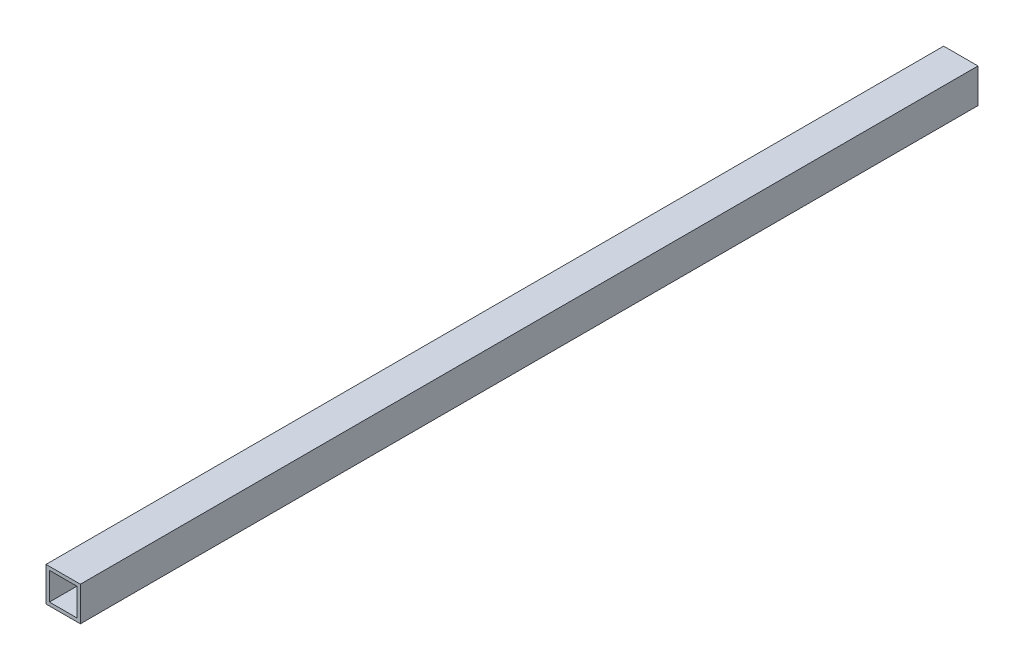
from build123d import *

# Parameters (mm, degrees)
SKETCH1_W           = 30
SKETCH1_H           = 30
SKETCH1_W_2         = 24
SKETCH1_H_2         = 24
BOSS_EXTRUDE2_DEPTH = 784


with BuildPart() as part:
    # Sketch1 → Boss-Extrude2 (new body)
    with BuildSketch(Plane.XY):
        with Locations((-1.115384615, 0.846363591)):
            Rectangle(SKETCH1_W, SKETCH1_H)
        with Locations((-1.115384615, 0.846363591)):
            Rectangle(SKETCH1_W_2, SKETCH1_H_2, mode=Mode.SUBTRACT)
    extrude(amount=BOSS_EXTRUDE2_DEPTH)


solid = part.part
